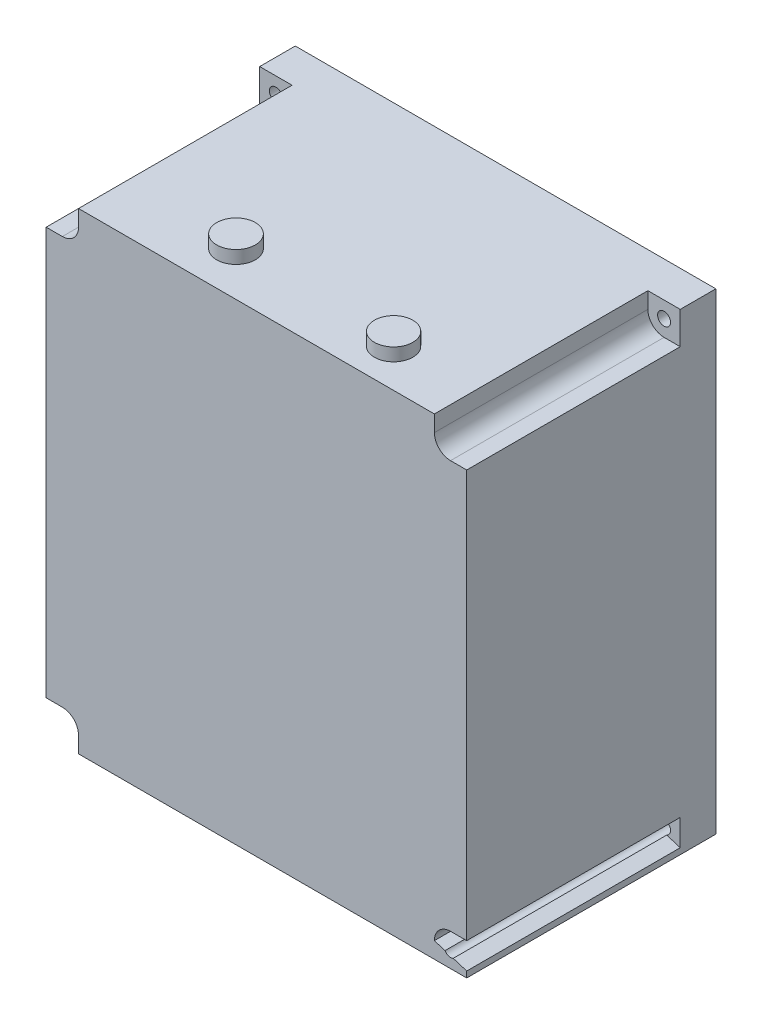
SolidWorks part; units mm, degrees
ref_plane "Front Plane" through (0, 0, 0) normal (0, 0, 1) x (1, 0, 0)
ref_plane "Top Plane" through (0, 0, 0) normal (0, 1, 0) x (1, 0, 0)
ref_plane "Right Plane" through (0, 0, 0) normal (1, 0, 0) x (0, 0, -1)
sketch "Sketch1" plane through (0, 0, 0) normal (0, 0, 1) x (1, 0, 0)
  line L1 (0, 0) -> (130, 0)
  line L2 (0, 0) -> (0, 146)
  line L3 (0, 146) -> (130, 146)
  line L4 (130, 0) -> (130, 146)
  line L5 (5, 141) -> (125, 141) construction
  line L6 (5, 141) -> (5, 5) construction
  line L7 (5, 5) -> (125, 5) construction
  line L8 (125, 141) -> (125, 5) construction
  circle A0 centre (5, 141) radius 2
  circle A1 centre (125, 141) radius 2
  circle A2 centre (125, 5) radius 2
  circle A3 centre (5, 5) radius 2
  dimension "D7" = 4
  dimension "D8" = 4
  dimension "D9" = 4
  dimension "D10" = 4
  dimension "D1" = 130
  dimension "D2" = 146
  dimension "D3" = 120
  dimension "D4" = 136
  dimension "D5" = 5
  dimension "D6" = 5
extrude "Boss-Extrude1" add sketch "Sketch1" along normal blind 77
sketch "Sketch3" plane through (0, 0, 77) normal (0, 0, 1) x (1, 0, 0)
  line L0 (120, 141) -> (120, 146)
  line L1 (130, 146) -> (0, 146) construction
  line L2 (120, 146) -> (146, 160)
  line L3 (146, 160) -> (130, 136)
  line L4 (130, 0) -> (130, 146) construction
  line L5 (130, 136) -> (125, 136)
  line L6 (10, 141) -> (10, 146)
  line L7 (10, 146) -> (0, 160)
  line L8 (0, 160) -> (0, 136)
  line L9 (0, 146) -> (0, 0) construction
  line L10 (0, 136) -> (5, 136)
  line L11 (10, 5) -> (10, 0)
  line L14 (10, 0) -> (0, 0)
  line L15 (0, 0) -> (0, 10)
  line L16 (0, 10) -> (5, 10)
  line L17 (120, 5) -> (136, 0)
  line L20 (136, 0) -> (146, 0)
  line L21 (146, 0) -> (130, 10)
  line L22 (130, 10) -> (125, 10)
  arc A0 (120, 141) -> (125, 136) centre (125, 141) ccw
  arc A3 (125, 10) -> (120, 5) centre (125, 5) ccw
  arc A6 (5, 136) -> (10, 141) centre (5, 141) ccw
  arc A7 (10, 5) -> (5, 10) centre (5, 5) ccw
  dimension "D1" = 10
  dimension "D2" = 10
extrude "Cut-Extrude2" cut sketch "Sketch3" against normal blind 66
sketch "Sketch4" plane through (0, 0, 0) normal (0, -1, 0) x (-1, 0, 0)
  circle A0 centre (-45.097, -63.4204) radius 5.9858
  circle A1 centre (-95.5649, -65.1647) radius 5.937
extrude "Boss-Extrude3" add sketch "Sketch4" against normal blind 150
